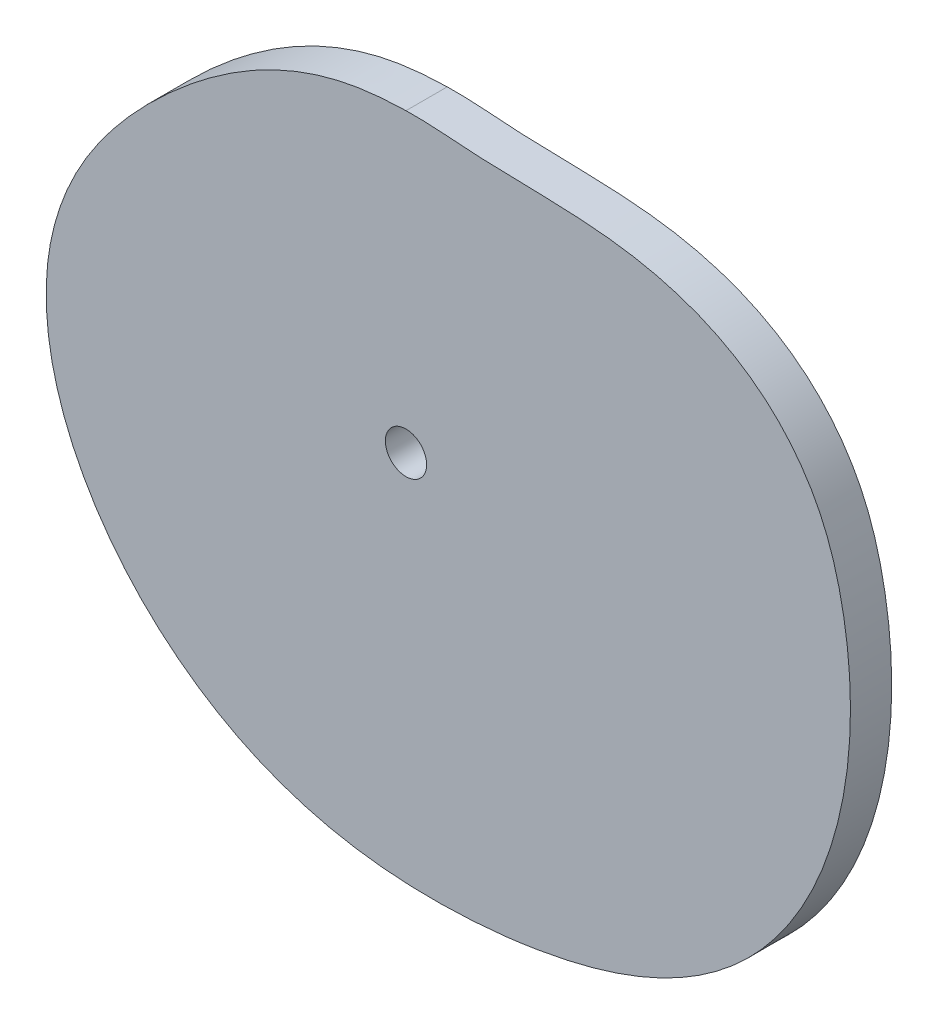
from build123d import *

# Parameters (mm, degrees)
SKETCH3_R           = 5
BOSS_EXTRUDE1_DEPTH = 10


with BuildPart() as part:
    # Sketch3 → Boss-Extrude1 (new body)
    with BuildSketch(Plane.XY):
        with BuildLine():
            add(Edge.make_bspline(
                [(32.098993714, -88.315090172), (24.790304353, -89.544235685), (8.555038023, -91.091547174), (-15.273114308, -89.578704931), (-40.023815861, -81.710972799), (-60.94601733, -67.639101592), (-77.368159975, -47.677546318), (-86.926677755, -25.321294301), (-88.005324434, -2.655584715), (-82.148845494, 15.87629255), (-73.16971112, 30.391235296), (-62.472045739, 42.448066508), (-50.147034888, 53.39154317), (-34.745911271, 63.872277011), (-17.483414176, 70.627368849), (-4.858503178, 71.704531936), (0, 71.816111973)],
                knots=[279.040236335, 279.040236335, 279.040236335, 279.040236335, 301.306934661, 327.990453655, 350.233781535, 378.703779471, 402.465795846, 427.140802183, 450.56156387, 469.038909602, 484.738658421, 501.583092965, 517.349838147, 534.207201166, 557.456049242, 572.073061531, 572.073061531, 572.073061531, 572.073061531], degree=3, weights=[1, 1, 1, 1, 1, 1, 1, 1, 1, 1, 1, 1, 1, 1, 1, 1, 1]))
            add(Edge.make_bspline(
                [(0, 71.816111973), (5.53148395, 71.943147639), (16.922952207, 70.74844157), (35.351697322, 70.647702193), (54.612200678, 69.567100223), (73.20185028, 64.366142209), (89.357471879, 54.264044334), (101.146128347, 38.708568873), (106.308485454, 20.393294593), (108.258687784, 1.415860382), (106.775560538, -19.572658629), (99.872309139, -42.357728983), (87.006382252, -61.853250376), (70.581747793, -75.404908213), (52.352597958, -83.965233493), (39.091960666, -87.139041564), (32.098993714, -88.315090172)],
                knots=[0, 0, 0, 0, 16.641703449, 34.322342536, 55.462542669, 74.476915764, 91.729365541, 111.905406957, 131.542163028, 148.207146298, 169.164435539, 194.407337177, 218.993051757, 238.231698049, 257.735419856, 279.040236335, 279.040236335, 279.040236335, 279.040236335], degree=3, weights=[1, 1, 1, 1, 1, 1, 1, 1, 1, 1, 1, 1, 1, 1, 1, 1, 1]))
        make_face()
        Circle(SKETCH3_R, mode=Mode.SUBTRACT)
    extrude(amount=BOSS_EXTRUDE1_DEPTH)


solid = part.part
